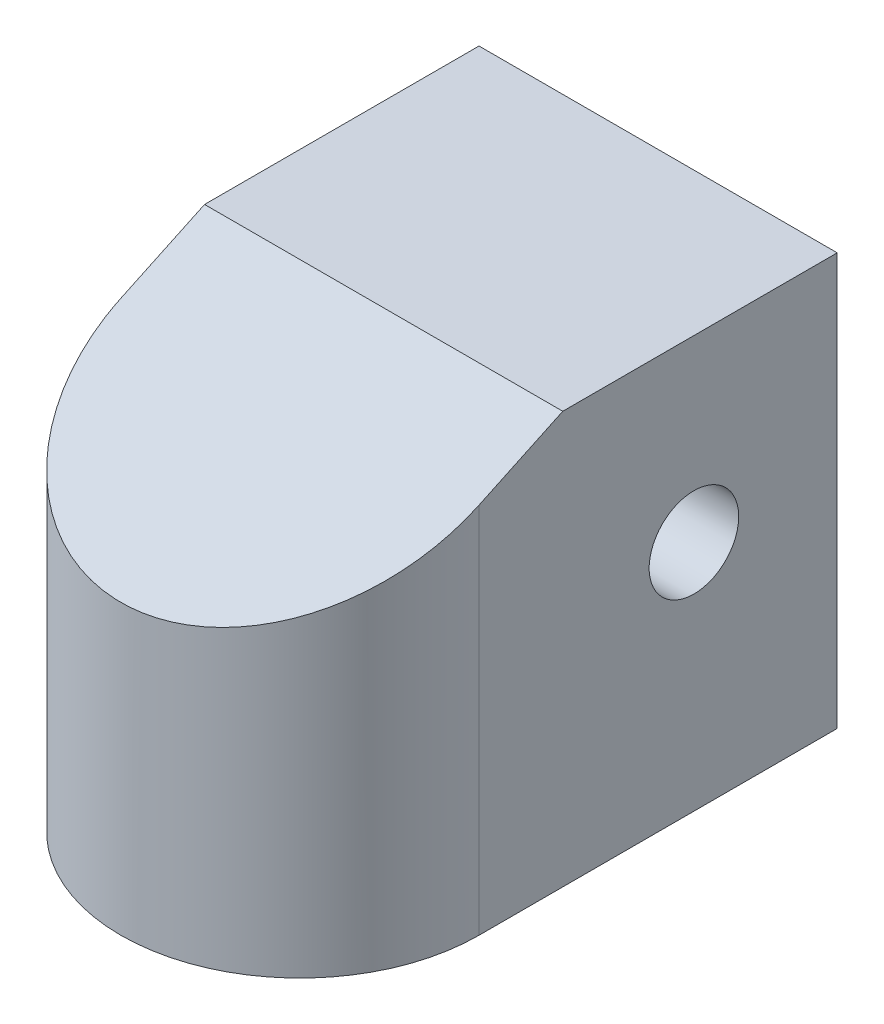
SolidWorks part; units mm, degrees
ref_plane "前视" through (0, 0, 0) normal (0, 0, 1) x (1, 0, 0)
ref_plane "上视" through (0, 0, 0) normal (0, 1, 0) x (1, 0, 0)
ref_plane "右视" through (0, 0, 0) normal (1, 0, 0) x (0, 0, -1)
sketch "草图1" plane through (0, 0, 0) normal (0, 1, 0) x (1, 0, 0)
  line L0 (-10, 0) -> (-10, 20)
  line L1 (-10, 20) -> (10, 20)
  line L2 (10, 20) -> (10, 0)
  arc A0 (-10, 0) -> (10, 0) centre (0, 0) ccw
  dimension "D1" = 20
  dimension "D2" = 20
extrude "凸台-拉伸1" add sketch "草图1" along normal blind 23
sketch "草图2" plane through (0, 0, 0) normal (0, -1, 0) x (1, 0, 0)
  circle A0 centre (0, 0) radius 2.5
extrude "切除-拉伸1" cut sketch "草图2" against normal blind 12
sketch "草图3" plane through (10, 0, 0) normal (1, 0, 0) x (0, 0, -1)
  line L0 (0, 23) -> (20, 23) construction
  line L1 (20, 23) -> (20, 0) construction
  circle A0 centre (12, 13) radius 2.5
  dimension "D1" = 10
  dimension "D2" = 8
extrude "切除-拉伸2" cut sketch "草图3" against normal blind 62
sketch "草图4" plane through (10, 0, 0) normal (1, 0, 0) x (0, 0, -1)
  line L0 (0, 23) -> (-10, 23)
  line L1 (-10, 23) -> (-10, 16.0969)
  line L2 (-10, 23) -> (-10, 0) construction
  line L3 (-10, 16.0969) -> (4.677, 23)
  line L4 (0, 23) -> (20, 23) construction
  line L5 (4.677, 23) -> (0, 23)
extrude "切除-拉伸3" cut sketch "草图4" against normal blind 26
